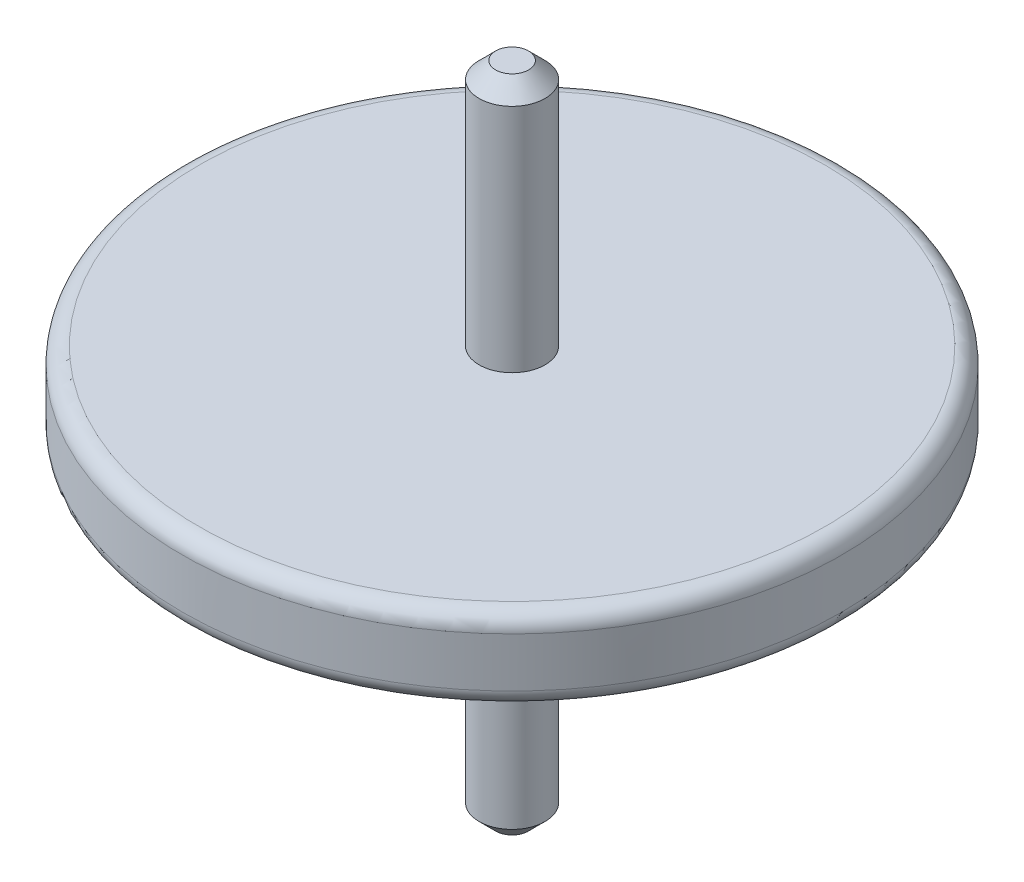
SolidWorks part; units mm, degrees
material "塑料"
ref_plane "Front Plane" through (0, 0, 0) normal (0, 0, 1) x (1, 0, 0)
ref_plane "Top Plane" through (0, 0, 0) normal (0, 1, 0) x (1, 0, 0)
ref_plane "Right Plane" through (0, 0, 0) normal (1, 0, 0) x (0, 0, -1)
sketch "Sketch1" plane through (0, 0, 0) normal (0, 0, 1) x (1, 0, 0)
  line L0 (0, 0) -> (0, 40) construction
  line L1 (0, 40) -> (-2, 40)
  line L2 (-2, 40) -> (-2, 25)
  line L3 (-2, 25) -> (-20, 25)
  line L4 (-20, 25) -> (-20, 20)
  line L5 (-20, 20) -> (-6, 20)
  line L6 (-6, 20) -> (-6, 15)
  line L7 (-6, 15) -> (-2, 15)
  line L8 (-2, 15) -> (-2, 0)
  line L9 (-2, 0) -> (0, 0)
  line L10 (0, 0) -> (0, 40)
  dimension "D1" = 40
  dimension "D2" = 5
  dimension "D3" = 4
  dimension "D4" = 4
  dimension "D5" = 12
  dimension "D6" = 40
  dimension "D7" = 5
revolve "Revolve1" add sketch "Sketch1" angle 360 about L0
chamfer "Chamfer1" distance 1 angle 45 2 edges at (0, 0, -2) (0, 40, -2)
fillet "Fillet1" radius 1 2 edges at (0, 20, -20) (0, 25, -20)
equation "\"TH\"= \"图号代号\""
equation "\"LJ\"= \"名称代号\""
